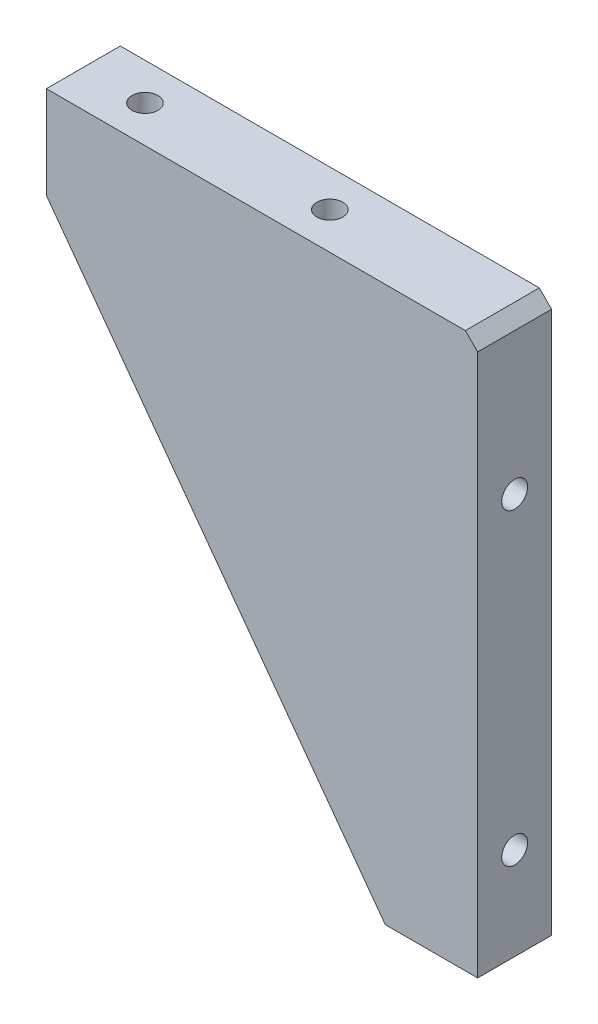
SolidWorks part; units mm, degrees
material "A6061"
ref_plane "前基準面" through (0, 0, 0) normal (0, 0, 1) x (1, 0, 0)
ref_plane "上基準面" through (0, 0, 0) normal (0, 1, 0) x (1, 0, 0)
ref_plane "右基準面" through (0, 0, 0) normal (1, 0, 0) x (0, 0, -1)
sketch "草图1" plane through (0, 0, 0) normal (0, 0, 1) x (1, 0, 0)
  line L0 (0, 0) -> (0, -90)
  line L1 (0, -90) -> (-15, -90)
  line L2 (-15, -90) -> (-70, -15)
  line L3 (-70, -15) -> (-70, 0)
  line L4 (-70, 0) -> (0, 0)
  dimension "D1" = 70
  dimension "D2" = 90
  dimension "D3" = 15
  dimension "D4" = 15
extrude "凸台-拉伸1" add sketch "草图1" along normal blind 12
hole_wizard "M5 螺纹孔1" positions "草图2" profile "草图3" tap size "M5" standard "GB"
sketch "草图2" plane through (0, 0, 0) normal (0, 1, 0) x (1, 0, 0)
  line L0 (0, -6) -> (-73.1743, -6) construction
  line L1 (0, -12) -> (0, 0) construction
  point P0 (-60, -6)
  point P2 (-30, -6)
  dimension "D1" = 30
  dimension "D2" = 30
sketch "草图3" plane through (-60, 0, 6) normal (1, 0, 0) x (0, 0, 1)
  line L0 (0, 0) -> (0, 13.6618)
  line L1 (0, 13.6618) -> (2.1, 12.4)
  line L2 (2.1, 12.4) -> (2.1, 0)
  line L5 (2.1, 0) -> (0, 0)
  line L10 (0, 13.6618) -> (-2.1, 12.4) construction
  line L11 (0, -6.35) -> (0, 107.95) construction
  dimension "螺纹孔钻头直径" = 4.2
  dimension "螺纹孔钻头深度" = 12.4
  dimension "导头角度" = 118
cosmetic thread "孔螺蚊线1" parameters "D1"=10, "D2"=5
cosmetic thread "孔螺蚊线2" parameters "D1"=10, "D2"=5
hole_wizard "M5 螺纹孔2" positions "草图4" profile "草图5" tap size "M5" standard "GB"
sketch "草图4" plane through (0, 0, 0) normal (1, 0, 0) x (0, 0, -1)
  line L0 (-6, -90) -> (-6, 3.634) construction
  line L1 (-12, -90) -> (0, -90) construction
  point P0 (-6, -75)
  point P2 (-6, -25)
  dimension "D1" = 15
  dimension "D2" = 50
sketch "草图5" plane through (0, -75, 6) normal (0, 1, 0) x (0, 0, -1)
  line L0 (0, 0) -> (0, 13.6618)
  line L1 (0, 13.6618) -> (2.1, 12.4)
  line L2 (2.1, 12.4) -> (2.1, 0)
  line L5 (2.1, 0) -> (0, 0)
  line L10 (0, 13.6618) -> (-2.1, 12.4) construction
  line L11 (0, -6.35) -> (0, 107.95) construction
  dimension "螺纹孔钻头直径" = 4.2
  dimension "螺纹孔钻头深度" = 12.4
  dimension "导头角度" = 118
cosmetic thread "孔螺蚊线3" parameters "D1"=10, "D2"=5
cosmetic thread "孔螺蚊线4" parameters "D1"=10, "D2"=5
chamfer "倒角1" distance 2 angle 45 1 edges at (0, 0, 6)
